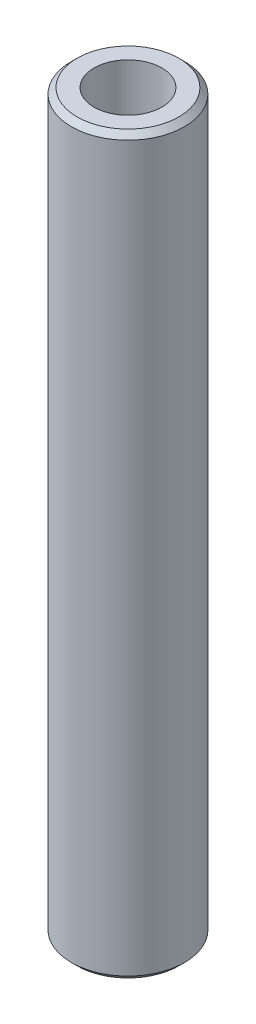
SolidWorks part; units mm, degrees
ref_plane "Front Plane" through (0, 0, 0) normal (0, 0, 1) x (1, 0, 0)
ref_plane "Top Plane" through (0, 0, 0) normal (0, 1, 0) x (1, 0, 0)
ref_plane "Right Plane" through (0, 0, 0) normal (1, 0, 0) x (0, 0, -1)
sketch "Sketch1" plane through (0, 0, 0) normal (0, 1, 0) x (1, 0, 0)
  circle A0 centre (0, 0) radius 5
  dimension "D1" = 10
extrude "Boss-Extrude1" add sketch "Sketch1" along normal blind 65
hole_wizard "Ø18.0 (18) Diameter Hole1" positions "Sketch3" profile "Sketch2" hole size "Ø18.0" standard "Ansi Metric"
sketch "Sketch3" plane through (0, 65, 0) normal (0, 1, 0) x (1, 0, 0)
  point P0 (0, 0)
sketch "Sketch2" plane through (0, 65, 0) normal (1, 0, 0) x (0, 0, 1)
  line L0 (0, 0) -> (0, 11.8026)
  line L1 (0, 11.8026) -> (3, 10)
  line L2 (3, 10) -> (3, 0)
  line L5 (3, 0) -> (0, 0)
  line L10 (0, 11.8026) -> (-3, 10) construction
  line L11 (0, -6.35) -> (0, 107.95) construction
  dimension "孔直径" = 6
  dimension "孔深度" = 10
  dimension "导头角度" = 118
ref_plane "Plane1" through (0, 32.5, 0) normal (0, 1, 0) x (1, 0, 0)
mirror "Mirror1" about plane through (0, 32.5, 0) normal (0, 1, 0) of "Ø18.0 (18) Diameter Hole1"
chamfer "Chamfer1" distance 0.5 angle 45 2 edges at (0, 65, 5) (0, 0, 5)
